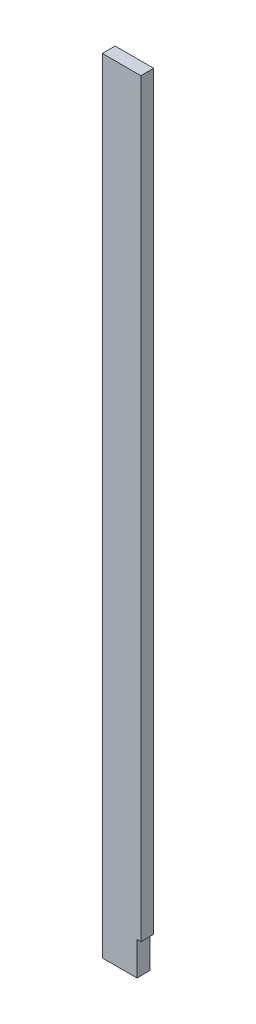
SolidWorks part; units mm, degrees
material "Plain Carbon Steel"
ref_plane "Front" through (0, 0, 0) normal (0, 0, 1) x (1, 0, 0)
ref_plane "Top" through (0, 0, 0) normal (0, 1, 0) x (1, 0, 0)
ref_plane "Right" through (0, 0, 0) normal (1, 0, 0) x (0, 0, -1)
sketch "Sketch1" plane through (0, 0, 0) normal (0, 0, 1) x (1, 0, 0)
  line L1 (0, 0) -> (30, 0)
  line L2 (0, 0) -> (0, -610)
  line L3 (0, -610) -> (30, -610)
  line L4 (30, 0) -> (30, -610)
  dimension "D1" = 610
  dimension "D2" = 30
extrude "Boss-Extrude1" add sketch "Sketch1" along normal blind 10
sketch "Sketch2" plane through (0, 0, 10) normal (0, 0, 1) x (1, 0, 0)
  line L1 (30, -610) -> (27, -610)
  line L2 (30, -610) -> (30, -584)
  line L3 (30, -584) -> (27, -584)
  line L4 (27, -610) -> (27, -584)
  dimension "D1" = 26
  dimension "D2" = 3
extrude "Cut-Extrude1" cut sketch "Sketch2" against normal blind 10
